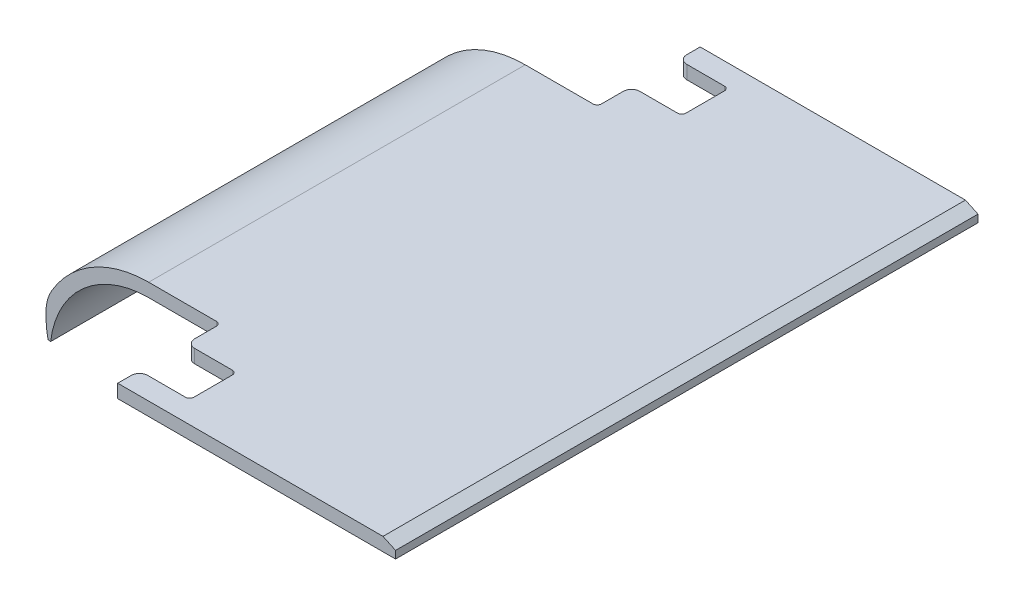
from build123d import *

# Parameters (mm, degrees)
BOSS_EXTRUDE1_DEPTH     = 348
CUT_EXTRUDE1_DEPTH      = 554.754458221
CUT_EXTRUDE1_DEPTH_BACK = 554.754458221
CUT_EXTRUDE3_DEPTH      = 717.846566568


with BuildPart() as part:
    # Sketch1 → Boss-Extrude1 (new, symmetric)
    with BuildSketch(Plane.XY):
        with BuildLine():
            Line((0, 0), (418, 0))
            Line((418, 0), (418, 9))
            Line((418, 9), (403, 16))
            Line((403, 16), (0, 16))
            ThreePointArc((0, 16), (-88.953996871, -17.784300428), (-133.053537704, -102.101694915))
            Line((-133.053537704, -102.101694915), (-117.166548127, -104))
            ThreePointArc((-117.166548127, -104), (-78.33262411, -29.750354108), (0, 0))
        make_face()
    extrude(amount=BOSS_EXTRUDE1_DEPTH, both=True)

    # Sketch2 → Cut-Extrude1 (cut, two sides: drawn at the far end of the back side and taken through both)
    with BuildSketch(Plane(origin=(0, 0, 0), x_dir=(1, 0, 0), z_dir=(0, 1, 0)).offset(-CUT_EXTRUDE1_DEPTH_BACK)):
        with BuildLine():
            Line((86, -256), (86, -230))
            ThreePointArc((86, -230), (84.535533906, -226.464466094), (81, -225))
            Line((81, -225), (-133.053537704, -225))
            Line((-133.053537704, -225), (-133.053537704, -348))
            Line((-133.053537704, -348), (86, -348))
            Line((86, -348), (86, -332))
            ThreePointArc((86, -332), (88.928932188, -324.928932188), (96, -322))
            Line((96, -322), (141, -322))
            ThreePointArc((141, -322), (144.535533906, -320.535533906), (146, -317))
            Line((146, -317), (146, -271))
            ThreePointArc((146, -271), (144.535533906, -267.464466094), (141, -266))
            Line((141, -266), (96, -266))
            ThreePointArc((96, -266), (88.928932188, -263.071067812), (86, -256))
        make_face()
        with BuildLine():
            Line((96, 322), (141, 322))
            ThreePointArc((141, 322), (144.535533906, 320.535533906), (146, 317))
            Line((146, 317), (146, 271))
            ThreePointArc((146, 271), (144.535533906, 267.464466094), (141, 266))
            Line((141, 266), (96, 266))
            ThreePointArc((96, 266), (88.928932188, 263.071067812), (86, 256))
            Line((86, 256), (86, 230))
            ThreePointArc((86, 230), (84.535533906, 226.464466094), (81, 225))
            Line((81, 225), (-133.053537704, 225))
            Line((-133.053537704, 225), (-133.053537704, 348))
            Line((-133.053537704, 348), (86, 348))
            Line((86, 348), (86, 332))
            ThreePointArc((86, 332), (88.928932188, 324.928932188), (96, 322))
        make_face()
    extrude(amount=CUT_EXTRUDE1_DEPTH + CUT_EXTRUDE1_DEPTH_BACK, mode=Mode.SUBTRACT)

    # Sketch3 → Cut-Extrude3 (cut, through all)
    with BuildSketch(Plane.XY.offset(225)):
        with BuildLine():
            Line((-120.305667655, -103.624912792), (-133.053537704, -102.101694915))
            ThreePointArc((-133.053537704, -102.101694915), (-127.139944881, -75.674659886), (-116.033703785, -50.976275946))
            ThreePointArc((-116.033703785, -50.976275946), (-120.754032763, -62.041779759), (-122.694651189, -73.9144745))
            ThreePointArc((-122.694651189, -73.9144745), (-122.404927497, -88.842445048), (-120.305667655, -103.624912792))
        make_face()
    extrude(amount=-CUT_EXTRUDE3_DEPTH, mode=Mode.SUBTRACT)


solid = part.part
